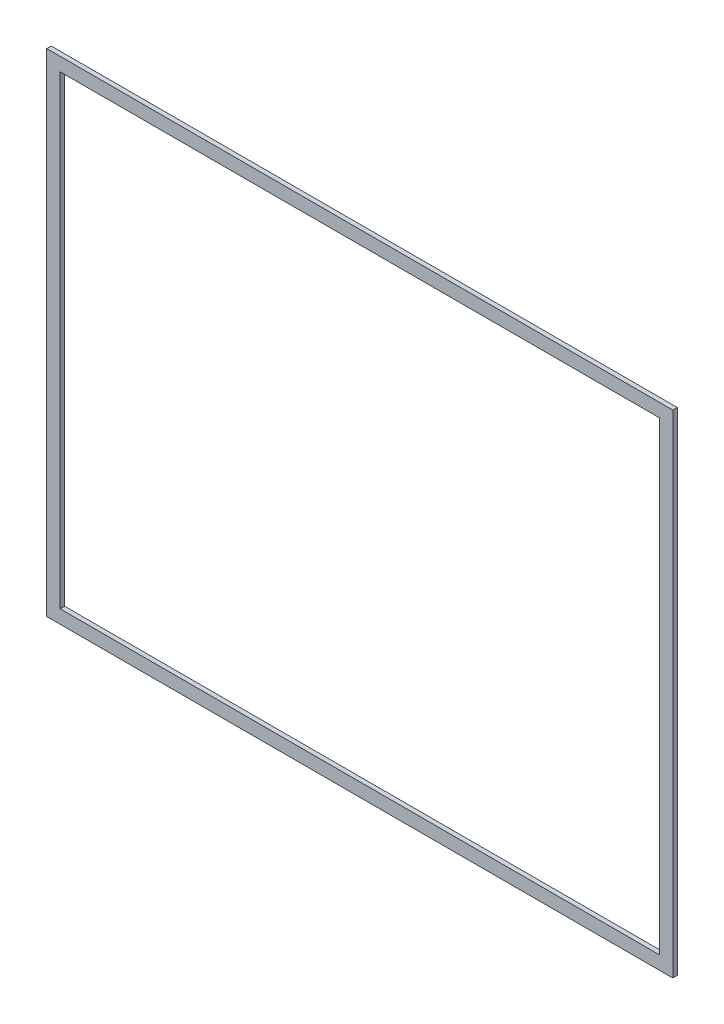
from build123d import *

# Parameters (mm, degrees)
SKETCH_1_W      = 140
SKETCH_1_H      = 110
SKETCH_1_W_2    = 134
SKETCH_1_H_2    = 104
EXTRUDE_1_DEPTH = 0.5


with BuildPart() as part:
    # 草图1 → 凸台-拉伸1 (new, symmetric)
    with BuildSketch(Plane.XY):
        Rectangle(SKETCH_1_W, SKETCH_1_H)
        Rectangle(SKETCH_1_W_2, SKETCH_1_H_2, mode=Mode.SUBTRACT)
    extrude(amount=EXTRUDE_1_DEPTH, both=True)


solid = part.part
